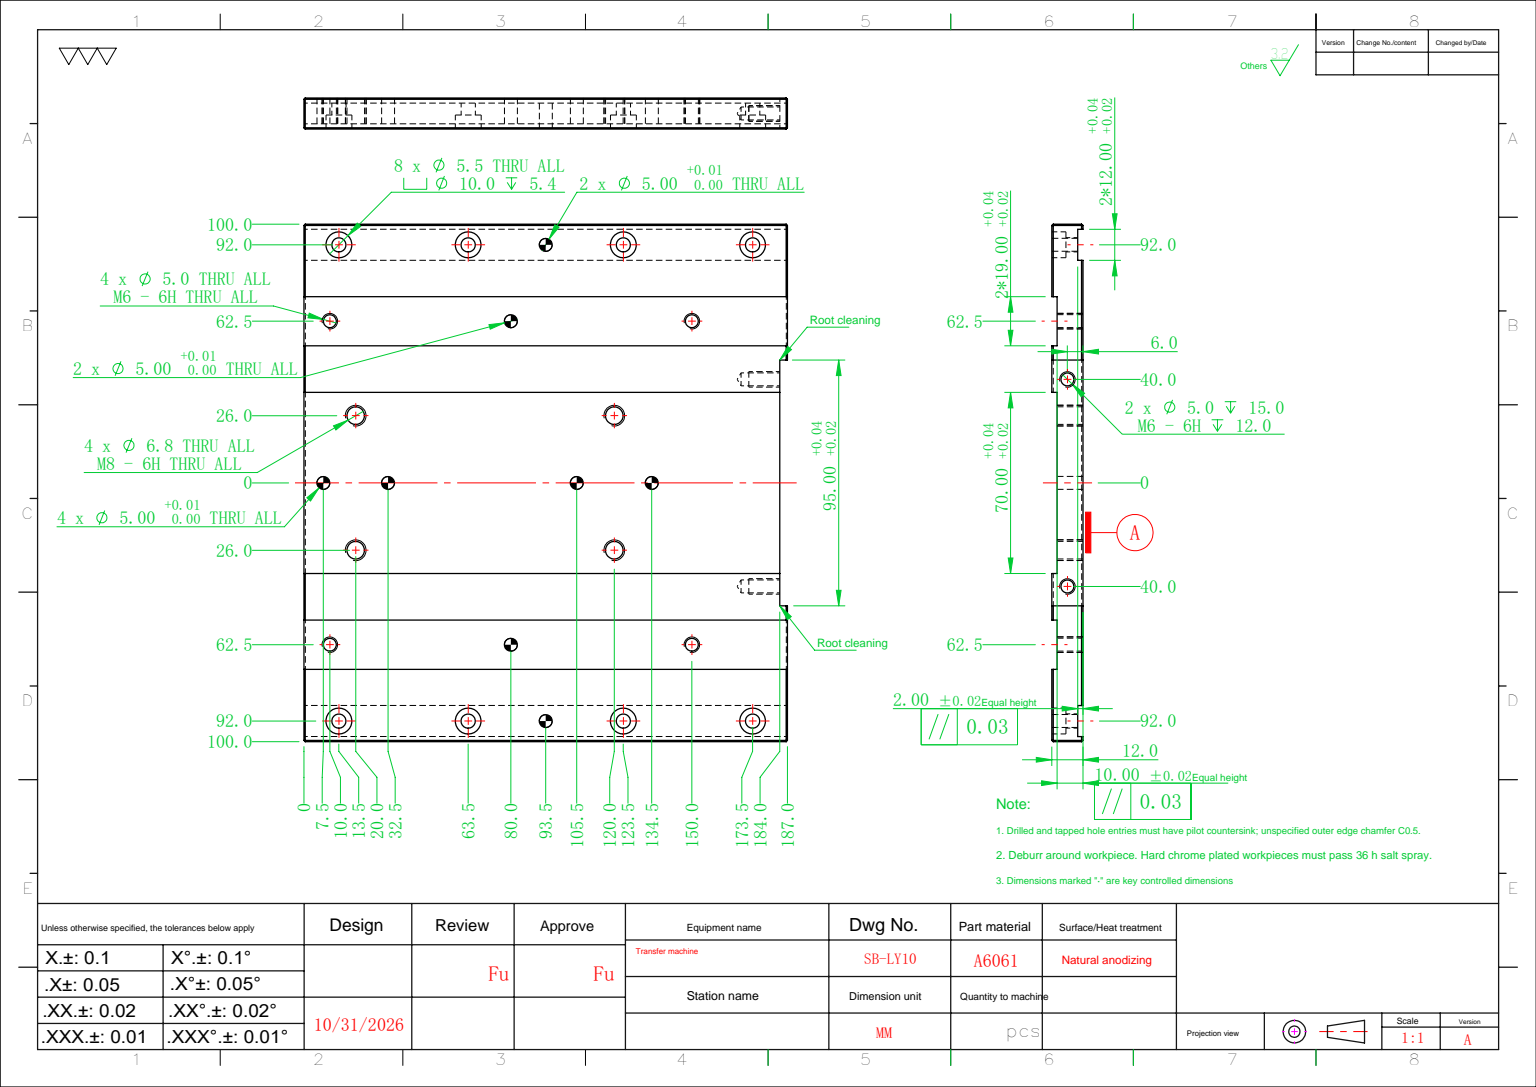
SolidWorks part; units mm, degrees
ref_plane "前视基准面" through (0, 0, 0) normal (0, 0, 1) x (1, 0, 0)
ref_plane "上视基准面" through (0, 0, 0) normal (0, 1, 0) x (1, 0, 0)
ref_plane "右视基准面" through (0, 0, 0) normal (1, 0, 0) x (0, 0, -1)
sketch "草图1" plane through (0, 0, 0) normal (0, 0, 1) x (1, 0, 0)
  line L1 (-100, -93.5) -> (100, -93.5)
  line L2 (-100, -93.5) -> (-100, 93.5)
  line L3 (-100, 93.5) -> (100, 93.5)
  line L4 (100, -93.5) -> (100, 93.5)
  line L5 (-100, -93.5) -> (100, 93.5) construction
  line L6 (-100, 93.5) -> (100, -93.5) construction
  point P0 (0, 0)
  dimension "D1" = 200
  dimension "D2" = 187
extrude "凸台-拉伸1" add sketch "草图1" along normal blind 12
sketch "草图4" plane through (0, 0, 0) normal (0, 0, -1) x (-1, 0, 0)
  line L0 (100, -93.5) -> (-100, -93.5) construction
  line L1 (-35, -93.5) -> (35, -93.5)
  line L2 (-35, -93.5) -> (-35, 93.5)
  line L3 (-35, 93.5) -> (35, 93.5)
  line L4 (35, -93.5) -> (35, 93.5)
  line L5 (-100, 93.5) -> (100, 93.5) construction
  line L6 (0, 93.5) -> (0, -110) construction
  dimension "D1" = 70
extrude "切除-拉伸3" cut sketch "草图4" against normal blind 2
sketch "草图5" plane through (0, 93.5, 0) normal (0, 1, 0) x (1, 0, 0)
  line L0 (100, -12) -> (-100, -12) construction
  line L1 (-98, -12) -> (-86, -12)
  line L2 (-98, -12) -> (-98, -10)
  line L3 (-98, -10) -> (-86, -10)
  line L4 (-86, -12) -> (-86, -10)
  line L5 (-92, -10) -> (-92, -17.0623) construction
  line L6 (-100, -12) -> (-100, 0) construction
  line L7 (0, 0) -> (0, -33.2156) construction
  line L8 (92, -10) -> (92, -17.0623) construction
  line L9 (86, -12) -> (86, -10)
  line L10 (98, -10) -> (86, -10)
  line L11 (98, -12) -> (98, -10)
  line L12 (98, -12) -> (86, -12)
  dimension "D1" = 12
  dimension "D2" = 8
  dimension "D3" = 2
extrude "切除-拉伸4" cut sketch "草图5" against normal through all
sketch "草图6" plane through (0, 93.5, 0) normal (0, 1, 0) x (1, 0, 0)
  line L0 (86, -12) -> (-86, -12) construction
  line L1 (47.5, -12) -> (-47.5, -12)
  line L2 (47.5, -12) -> (47.5, 0)
  line L3 (47.5, 0) -> (-47.5, 0)
  line L4 (-47.5, -12) -> (-47.5, 0)
  line L5 (-35, 0) -> (-100, 0) construction
  line L10 (0, 0) -> (0, -28.6653) construction
  dimension "D1" = 95
extrude "切除-拉伸5" cut sketch "草图6" against normal blind 3
hole_wizard "M6 螺纹孔1" positions "草图7" profile "草图8" tap size "M6" standard "ISO"
sketch "草图7" plane through (0, 90.5, 0) normal (0, 1, 0) x (1, 0, 0)
  line L0 (0, -12) -> (0, 8.4263) construction
  line L1 (-47.5, -12) -> (47.5, -12) construction
  point P0 (-40, -6)
  point P3 (40, -6)
  dimension "D1" = 80
  dimension "D2" = 6
sketch "草图8" plane through (-40, 90.5, 6) normal (1, 0, 0) x (0, 0, 1)
  line L0 (0, 0) -> (0, 16.5022)
  line L1 (0, 16.5022) -> (2.5, 15)
  line L2 (2.5, 15) -> (2.5, 0)
  line L5 (2.5, 0) -> (0, 0)
  line L10 (0, 16.5022) -> (-2.5, 15) construction
  line L11 (0, -6.35) -> (0, 107.95) construction
  dimension "螺纹孔钻头直径" = 5
  dimension "螺纹孔钻头深度" = 15
  dimension "导头角度" = 118
cosmetic thread "孔螺蚊线1" parameters "D1"=12, "D2"=6
cosmetic thread "孔螺蚊线2" parameters "D1"=12, "D2"=6
sketch "草图9" plane through (0, 0, 0) normal (0, 0, -1) x (-1, 0, 0)
  line L0 (-35, -93.5) -> (-100, -93.5) construction
  line L1 (-53, -93.5) -> (-72, -93.5)
  line L2 (-53, -93.5) -> (-53, 93.5)
  line L3 (-53, 93.5) -> (-72, 93.5)
  line L4 (-72, -93.5) -> (-72, 93.5)
  line L5 (-100, 93.5) -> (-47.5, 93.5) construction
  line L8 (0, 0) -> (0, 143.7921) construction
  line L9 (72, -93.5) -> (72, 93.5)
  line L10 (53, 93.5) -> (72, 93.5)
  line L11 (53, -93.5) -> (53, 93.5)
  line L12 (53, -93.5) -> (72, -93.5)
  line L13 (-62.5, 93.5) -> (-62.5, -120.0031) construction
  line L14 (62.5, 93.5) -> (62.5, -123.6896) construction
  dimension "D1" = 125
  dimension "D2" = 19
extrude "切除-拉伸6" cut sketch "草图9" against normal up to surface (2 mm away) up to face at (0, -1.5, 2)
hole_wizard "M8 螺纹孔1" positions "草图10" profile "草图11" tap size "M8" standard "ISO" end condition through all
sketch "草图10" plane through (0, 0, 0) normal (0, 0, -1) x (-1, 0, 0)
  line L0 (0, 0) -> (0, -140.4896) construction
  line L2 (86, -93.5) -> (-86, -93.5) construction
  point P0 (26, -73.5)
  point P4 (-26, -73.5)
  point P18 (26, 26.5)
  point P21 (-26, 26.5)
  dimension "D1" = 52
  dimension "D2" = 20
  dimension "D3" = 100
sketch "草图11" plane through (-26, -73.5, 0) normal (1, 0, 0) x (0, 1, 0)
  line L0 (0, 0) -> (0, 12)
  line L1 (0, 12) -> (3.4, 12)
  line L2 (3.4, 12) -> (3.4, 0)
  line L5 (3.4, 0) -> (0, 0)
  line L11 (0, -6.35) -> (0, 107.95) construction
  dimension "通孔螺纹孔钻头直径" = 6.8
  dimension "通孔螺纹孔钻头深度" = 12
cosmetic thread "孔螺蚊线3" parameters "D2"=8
cosmetic thread "孔螺蚊线4" parameters "D2"=8
cosmetic thread "孔螺蚊线5" parameters "D2"=8
cosmetic thread "孔螺蚊线6" parameters "D2"=8
hole_wizard "大小mm 暗销孔0" positions "草图12" profile "草图13" hole size "Ø5.0" standard "ISO" end condition through all
sketch "草图12" plane through (0, 0, 2) normal (0, 0, -1) x (-1, 0, 0)
  line L0 (0, -93.5) -> (0, 90.5) construction
  line L1 (-35, -93.5) -> (35, -93.5) construction
  line L2 (-35, 90.5) -> (35, 90.5) construction
  circle A0 centre (26, -73.5) radius 3.4 construction
  circle A1 centre (26, 26.5) radius 3.4 construction
  point P0 (0, -86)
  point P2 (0, -61)
  point P20 (0, 12)
  point P22 (0, 41)
  dimension "D2" = 12.5
  dimension "D1" = 12.5
  dimension "D3" = 14.5
  dimension "D4" = 14.5
sketch "草图13" plane through (0, -86, 2) normal (1, 0, 0) x (0, 1, 0)
  line L0 (0, 0) -> (0, 10)
  line L1 (0, 10) -> (2.5, 10)
  line L2 (2.5, 10) -> (2.5, 0)
  line L5 (2.5, 0) -> (0, 0)
  line L11 (0, -6.35) -> (0, 107.95) construction
  dimension "通孔孔直径" = 5
  dimension "通孔孔深度" = 10
hole_wizard "M6 螺纹孔2" positions "草图14" profile "草图15" tap size "M6" standard "ISO" end condition through all
sketch "草图14" plane through (0, 0, 2) normal (0, 0, -1) x (-1, 0, 0)
  line L0 (0, 0) -> (0, -116.6414) construction
  line L2 (86, -93.5) -> (-86, -93.5) construction
  point P0 (62.5, -83.5)
  point P3 (62.5, 56.5)
  point P6 (-62.5, 56.5)
  point P9 (-62.5, -83.5)
  dimension "D1" = 125
  dimension "D2" = 10
  dimension "D3" = 140
sketch "草图15" plane through (-62.5, -83.5, 2) normal (1, 0, 0) x (0, 1, 0)
  line L0 (0, 0) -> (0, 10)
  line L1 (0, 10) -> (2.5, 10)
  line L2 (2.5, 10) -> (2.5, 0)
  line L5 (2.5, 0) -> (0, 0)
  line L11 (0, -6.35) -> (0, 107.95) construction
  dimension "通孔螺纹孔钻头直径" = 5
  dimension "通孔螺纹孔钻头深度" = 10
cosmetic thread "孔螺蚊线11" parameters "D2"=6
cosmetic thread "孔螺蚊线12" parameters "D2"=6
cosmetic thread "孔螺蚊线13" parameters "D2"=6
cosmetic thread "孔螺蚊线14" parameters "D2"=6
hole_wizard "大小mm 暗销孔1" positions "草图16" profile "草图17" hole size "Ø5.0" standard "ISO" end condition through all
sketch "草图16" plane through (0, 0, 2) normal (0, 0, -1) x (-1, 0, 0)
  line L0 (62.5, -83.5) -> (62.5, 56.5) construction
  line L2 (-62.5, -83.5) -> (-62.5, 56.5) construction
  point P0 (-62.5, -13.5)
  point P2 (62.5, -13.5)
sketch "草图17" plane through (62.5, -13.5, 2) normal (1, 0, 0) x (0, 1, 0)
  line L0 (0, 0) -> (0, 10)
  line L1 (0, 10) -> (2.5, 10)
  line L2 (2.5, 10) -> (2.5, 0)
  line L5 (2.5, 0) -> (0, 0)
  line L11 (0, -6.35) -> (0, 107.95) construction
  dimension "通孔孔直径" = 5
  dimension "通孔孔深度" = 10
hole_wizard "M5 六角凹头螺钉的柱形沉头孔1" positions "草图18" profile "草图19" counterbore size "M5" standard "ISO" end condition through all
sketch "草图18" plane through (0, 0, 0) normal (0, 0, -1) x (-1, 0, 0)
  line L0 (-92, -93.5) -> (-92, 93.5) construction
  line L1 (-98, -93.5) -> (-86, -93.5) construction
  line L2 (-98, 93.5) -> (-86, 93.5) construction
  line L4 (-92, 0) -> (129.814, 0) construction
  line L6 (0, 0) -> (0, -109.5362) construction
  point P0 (-92, 80)
  point P2 (-92, -80)
  point P6 (-92, 30)
  point P11 (-92, -30)
  point P34 (92, -30)
  point P35 (92, 30)
  point P36 (92, -80)
  point P37 (92, 80)
  dimension "D1" = 60
  dimension "D2" = 160
sketch "草图19" plane through (92, 80, 0) normal (1, 0, 0) x (0, 1, 0)
  line L0 (0, 0) -> (0, 12)
  line L1 (0, 12) -> (2.75, 12)
  line L3 (2.75, 12) -> (2.75, 5.4)
  line L4 (2.75, 5.4) -> (5, 5.4)
  line L5 (5, 5.4) -> (5, 0)
  line L7 (5, 0) -> (0, 0)
  line L11 (0, -6.35) -> (0, 107.95) construction
  dimension "通孔孔直径" = 5.5
  dimension "通孔孔深度" = 12
  dimension "柱形沉头孔直径" = 10
  dimension "柱形沉头孔深度" = 5.4
hole_wizard "大小mm 暗销孔2" positions "草图20" profile "草图21" hole size "Ø5.0" standard "ISO" end condition through all
sketch "草图20" plane through (0, 0, 0) normal (0, 0, -1) x (-1, 0, 0)
  line L0 (92, 30) -> (92, -30) construction
  line L2 (0, 0) -> (0, 120.8639) construction
  point P0 (92, 0)
  point P15 (-92, 0)
sketch "草图21" plane through (-92, 0, 0) normal (1, 0, 0) x (0, 1, 0)
  line L0 (0, 0) -> (0, 12)
  line L1 (0, 12) -> (2.5, 12)
  line L2 (2.5, 12) -> (2.5, 0)
  line L5 (2.5, 0) -> (0, 0)
  line L11 (0, -6.35) -> (0, 107.95) construction
  dimension "通孔孔直径" = 5
  dimension "通孔孔深度" = 12
chamfer "倒角1" distance 0.5 angle 45 23 edges at (-44, -93.5, 0) (0, -93.5, 12) (44, -93.5, 0) (-100, 0, 12) (-99, -93.5, 12) (-100, -93.5, 6) (-86, -93.5, 0) (-100, 0, 0) (-99, 93.5, 12) (-100, 93.5, 6) (-86, 93.5, 0) (-66.75, 93.5, 12) (-50.25, 93.5, 0) (50.25, 93.5, 0) (66.75, 93.5, 12) (100, -93.5, 6) (99, -93.5, 12) (100, 0, 12) (99, 93.5, 12) (100, 93.5, 6) (86, -93.5, 0) (100, 0, 0) (86, 93.5, 0)
